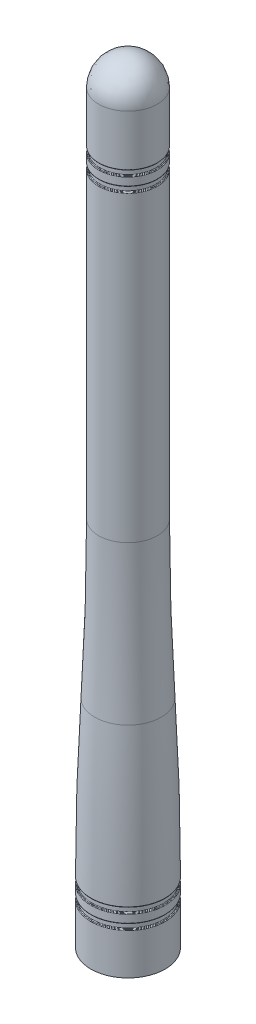
SolidWorks part; units mm, degrees
material "ABS"
ref_plane "Front Plane" through (0, 0, 0) normal (0, 0, 1) x (1, 0, 0)
ref_plane "Top Plane" through (0, 0, 0) normal (0, 1, 0) x (1, 0, 0)
ref_plane "Right Plane" through (0, 0, 0) normal (1, 0, 0) x (0, 0, -1)
sketch "Sketch2" plane through (0, 0, 0) normal (0, 0, 1) x (1, 0, 0)
  line L0 (-5, 0) -> (-5, 5.6098)
  line L1 (-3.95, 90.8) -> (-3.95, 50)
  line L2 (-3.8, 0) -> (-5, 0)
  line L3 (-4.8, 5.6098) -> (-5, 5.6098)
  line L4 (-4.8, 6.3098) -> (-5, 6.3098)
  line L5 (-4.8, 7.5098) -> (-5, 7.5098)
  line L6 (-4.8, 8.2098) -> (-5, 8.2098)
  line L7 (-4.8, 5.6098) -> (-4.8, 6.3098)
  line L8 (-4.8, 7.5098) -> (-4.8, 8.2098)
  line L9 (-5, 8.2098) -> (-5, 25) construction
  line L10 (-5, 6.3098) -> (-5, 7.5098)
  line L11 (-3.75, 93.4) -> (-3.95, 93.4)
  line L12 (-3.75, 92.7) -> (-3.95, 92.7)
  line L13 (-3.75, 91.5) -> (-3.95, 91.5)
  line L14 (-3.75, 90.8) -> (-3.95, 90.8)
  line L15 (-3.75, 90.8) -> (-3.75, 91.5)
  line L16 (-3.95, 93.4) -> (-3.95, 100.3)
  line L17 (-3.75, 92.7) -> (-3.75, 93.4)
  line L18 (-3.95, 91.5) -> (-3.95, 92.7)
  line L19 (0, 104.1997) -> (0, 100.3)
  line L20 (0, 110.0884) -> (0, -10.7959) construction
  line L21 (-3.8, 22.4788) -> (-3.8, 4)
  line L22 (-2.9521, 100.3) -> (-2.9521, 50)
  line L23 (-3.8, 1.5) -> (-4, 1.5)
  line L24 (-2.9521, 100.3) -> (0, 100.3)
  line L25 (-4, 1.5) -> (-4, 2)
  line L26 (-4, 2) -> (-3.8, 2)
  line L27 (-3.8, 2.5) -> (-4, 2.5)
  line L28 (-4, 2.5) -> (-4, 3)
  line L29 (-4, 3) -> (-3.8, 3)
  line L30 (-3.8, 3.5) -> (-4, 3.5)
  line L31 (-4, 3.5) -> (-4, 4)
  line L32 (-4, 4) -> (-3.8, 4)
  line L33 (-3.8, 3.5) -> (-3.8, 3)
  line L34 (-3.8, 2.5) -> (-3.8, 2)
  line L35 (-3.8, 1.5) -> (-3.8, 0)
  arc A0 (0, 104.1997) -> (-3.95, 100.3) centre (-0.05, 100.3) ccw
  arc A1 (-2.9521, 50) -> (-3.7431, 24.3255) centre (-420.0288, 50) cw
  arc A2 (-3.95, 50) -> (-4.475, 29.1048) centre (-420.0288, 50) cw
  arc A3 (-5, 8.2098) -> (-4.475, 29.1048) centre (411.0751, 8.2098) cw
  arc A4 (-3.7431, 24.3255) -> (-3.8, 22.4788) centre (26.2, 22.4788) ccw
  point P33 (-420.0288, 50)
  point P35 (-2.45, 50)
  point P36 (-3.8, 23.4191)
  dimension "D2" = 7.9
  dimension "D15" = 10
  dimension "D16" = 3.9
  dimension "D17" = 30
  dimension "D3" = 50
  dimension "D9" = 8.95
  dimension "D18" = 7.6
  dimension "D19" = 1.5
  dimension "D1" = 10
  dimension "D4" = 1.2
  dimension "D5" = 0.7
  dimension "D6" = 0.2
  dimension "D10" = 25
  dimension "D11" = 5.6098
  dimension "D12" = 1.2
  dimension "D13" = 0.7
  dimension "D14" = 0.2
  dimension "D20" = 0.2
  dimension "D21" = 0.5
  dimension "D22" = 0.5
  dimension "D23" = 0.2
  dimension "D24" = 0.5
  dimension "D25" = 0.5
  dimension "D26" = 0.5
revolve "Revolve1" add sketch "Sketch2" angle 360 about L20
fillet "Fillet1" radius 0.08 16 edges at (0, 90.8, 3.75) (0, 90.8, 3.95) (0, 91.5, 3.95) (0, 91.5, 3.75) (0, 92.7, 3.75) (0, 92.7, 3.95) (0, 93.4, 3.75) (0, 93.4, 3.95) (0, 5.6098, 5) (0, 5.6098, 4.8) (0, 6.3098, 5) (0, 6.3098, 4.8) (0, 7.5098, 5) (0, 7.5098, 4.8) (0, 8.2098, 4.8) (0, 8.2098, 5)
